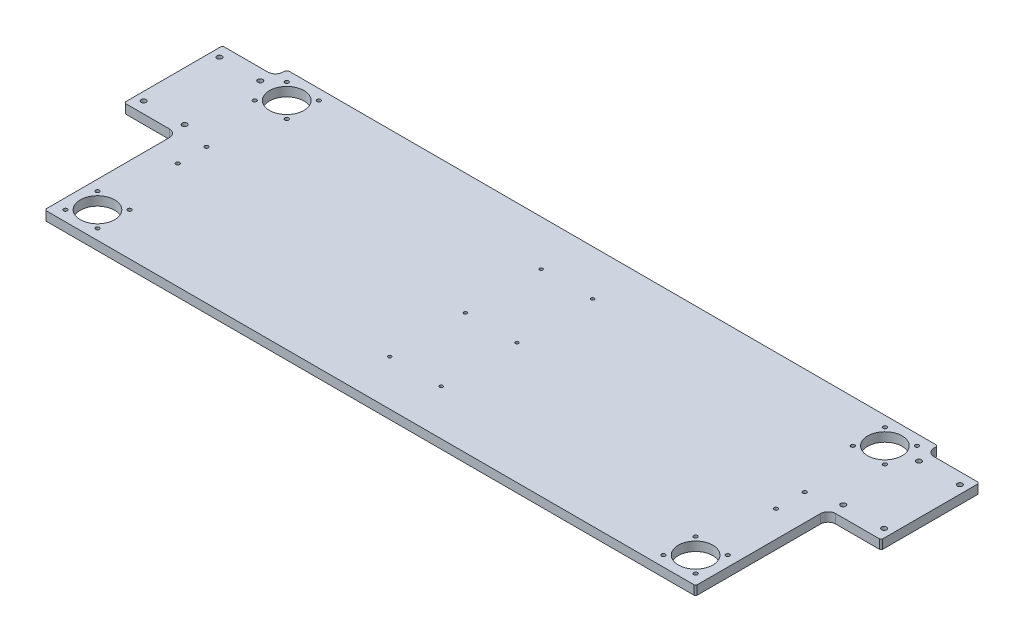
from build123d import *

# Parameters (mm, degrees)
SKETCH_1_W                = 1000
SKETCH_1_H                = 12
EXTRUDE_1_DEPTH           = 320
HOLE_WIZARD_M5_1_D        = 4.2
HOLE_WIZARD_25_0_45_5_1_D = 45.5
CUT_EXTRUDE_2_DEPTH       = 12
HOLE_WIZARD_2_D           = 6.6
HOLE_WIZARD_2_CBORE_D     = 11
HOLE_WIZARD_2_CBORE_DEPTH = 6.8
CHAMFER_1_SIZE            = 2
HOLE_WIZARD_M6_1_D        = 5
HOLE_WIZARD_M6_2_D        = 5


with BuildPart() as part:
    # 草图1 → 凸台-拉伸1 (new body)
    with BuildSketch(Plane.XY):
        Rectangle(SKETCH_1_W, SKETCH_1_H)
    extrude(amount=EXTRUDE_1_DEPTH)

    # M5 螺纹孔1 (through all)
    with Locations(Plane(origin=(0, -6, 0), x_dir=(-1, 0, 0), z_dir=(0, -1, 0))):
        with Locations((34, -60), (34, -260), (-34, -260), (34, -160), (-34, -160), (-34, -60)):
            Hole(HOLE_WIZARD_M5_1_D / 2)

    # Ø25.0 (45.5) 直径孔1 (through all)
    with Locations(Plane(origin=(0, 6, 0), x_dir=(1, 0, 0), z_dir=(0, 1, 0))):
        with Locations((395, -285), (395, -35), (-395, -35), (-395, -285)):
            Hole(HOLE_WIZARD_25_0_45_5_1_D / 2)

    # 草图22 → 切除-拉伸2 (cut)
    with BuildSketch(Plane.XZ.offset(6)):
        with BuildLine():
            Line((500, 320), (430, 320))
            Line((430, 320), (430, 155))
            ThreePointArc((430, 155), (432.928932188, 147.928932188), (440, 145))
            Line((440, 145), (500, 145))
            Line((500, 145), (500, 320))
        make_face()
        with BuildLine():
            Line((-430, 320), (-430, 155))
            ThreePointArc((-430, 155), (-432.928932188, 147.928932188), (-440, 145))
            Line((-440, 145), (-500, 145))
            Line((-500, 145), (-500, 320))
            Line((-500, 320), (-430, 320))
        make_face()
        with BuildLine():
            Line((-430, 0), (-430, 5))
            ThreePointArc((-430, 5), (-432.928932188, 12.071067812), (-440, 15))
            Line((-440, 15), (-500, 15))
            Line((-500, 15), (-500, 0))
            Line((-500, 0), (-430, 0))
        make_face()
        with BuildLine():
            Line((500, 0), (430, 0))
            Line((430, 0), (430, 5))
            ThreePointArc((430, 5), (432.928932188, 12.071067812), (440, 15))
            Line((440, 15), (500, 15))
            Line((500, 15), (500, 0))
        make_face()
    extrude(amount=-CUT_EXTRUDE_2_DEPTH, mode=Mode.SUBTRACT)

    # 打孔尺寸(%根据)内六角圆柱头螺钉的类型2 (through all)
    with Locations(Plane.XZ.offset(6)):
        with Locations((489, 130), (489, 30), (435, 30), (435, 130), (-435, 130), (-435, 30), (-489, 30), (-489, 130)):
            CounterBoreHole(HOLE_WIZARD_2_D / 2, HOLE_WIZARD_2_CBORE_D / 2, HOLE_WIZARD_2_CBORE_DEPTH)

    # 倒角1
    chamfer_1_edges = [part.edges().sort_by_distance(p)[0] for p in [
        (-430, 0, 0),
        (-500, 0, 15),
        (500, 0, 145),
        (430, 0, 320),
        (-500, 0, 145),
        (-430, 0, 320),
        (500, 0, 15),
        (430, 0, 0),
    ]]
    chamfer(chamfer_1_edges, length=CHAMFER_1_SIZE)

    # M6 螺纹孔1 (through all)
    with Locations(Plane(origin=(0, 6, 0), x_dir=(1, 0, 0), z_dir=(0, 1, 0))):
        with Locations((-395, -141), (-395, -179), (395, -179), (395, -141)):
            Hole(HOLE_WIZARD_M6_1_D / 2)

    # M6 螺纹孔2 (through all)
    with Locations(Plane(origin=(0, -6, 0), x_dir=(-1, 0, 0), z_dir=(0, -1, 0))):
        with Locations((-416.213203436, -263.786796564), (-373.786796564, -263.786796564), (-373.786796564, -306.213203436), (-416.213203436, -306.213203436), (373.786796564, -263.786796564), (416.213203436, -263.786796564), (416.213203436, -306.213203436), (373.786796564, -306.213203436), (373.786796564, -13.786796564), (416.213203436, -13.786796564), (416.213203436, -56.213203436), (373.786796564, -56.213203436), (-416.213203436, -13.786796564), (-373.786796564, -13.786796564), (-373.786796564, -56.213203436), (-416.213203436, -56.213203436)):
            Hole(HOLE_WIZARD_M6_2_D / 2)


solid = part.part
